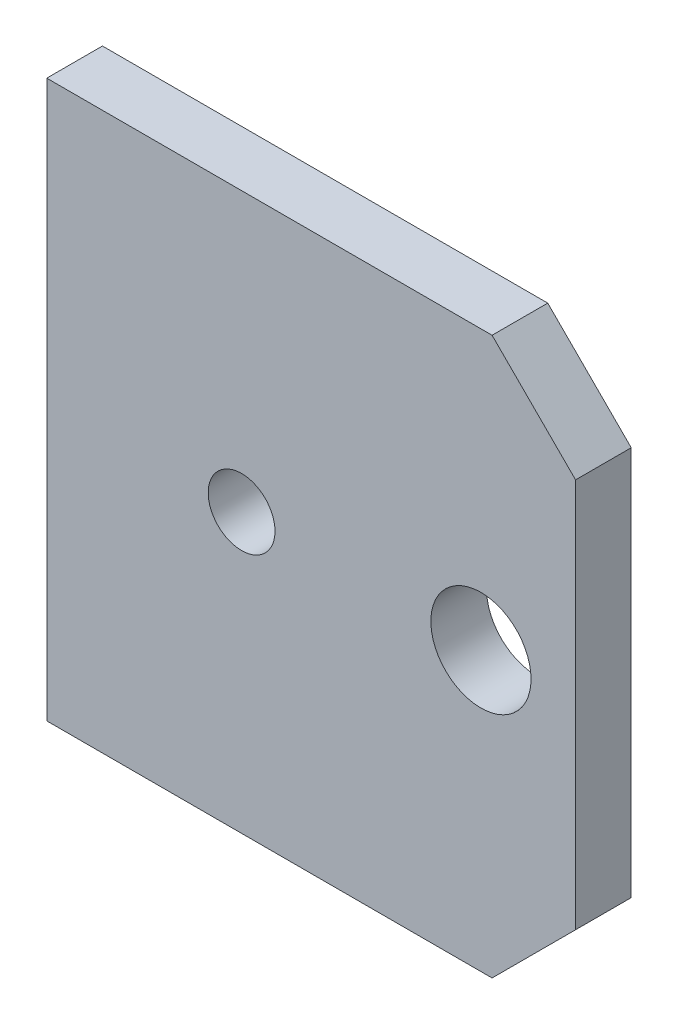
from build123d import *

# Parameters (mm, degrees)
SKETCH_1_R      = 6
SKETCH_1_R_2    = 9
EXTRUDE_1_DEPTH = 10


with BuildPart() as part:
    # 草图1 → 凸台-拉伸1 (new body)
    with BuildSketch(Plane.XY):
        Polygon((47.5, 35), (32.5, 50), (-47.5, 50), (-47.5, -50), (32.5, -50), (47.5, -35), align=None)
        with Locations((-12.5, 0)):
            Circle(SKETCH_1_R, mode=Mode.SUBTRACT)
        with Locations((30.5, 0)):
            Circle(SKETCH_1_R_2, mode=Mode.SUBTRACT)
    extrude(amount=EXTRUDE_1_DEPTH)


solid = part.part
